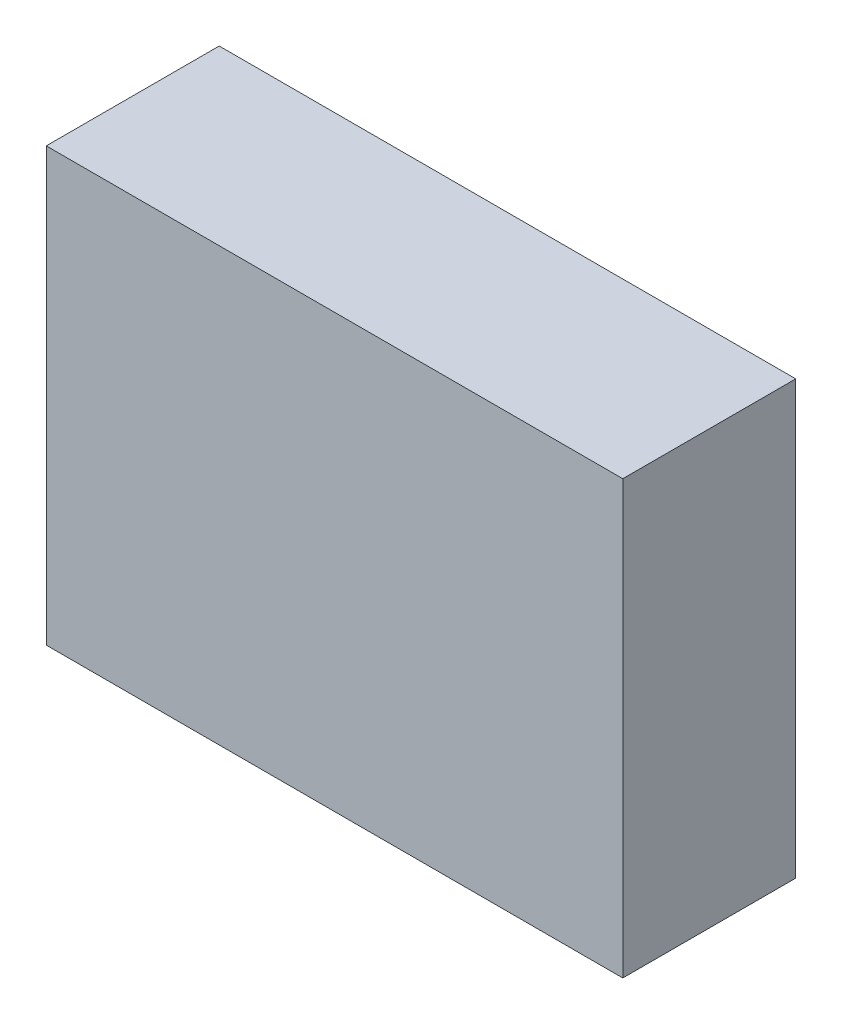
SolidWorks part; units mm, degrees
ref_plane "前视基准面" through (0, 0, 0) normal (0, 0, 1) x (1, 0, 0)
ref_plane "上视基准面" through (0, 0, 0) normal (0, 1, 0) x (1, 0, 0)
ref_plane "右视基准面" through (0, 0, 0) normal (1, 0, 0) x (0, 0, -1)
sketch "草图1" plane through (0, 0, 0) normal (0, 0, 1) x (1, 0, 0)
  line L1 (-20, -15) -> (20, -15)
  line L2 (-20, -15) -> (-20, 15)
  line L3 (-20, 15) -> (20, 15)
  line L4 (20, -15) -> (20, 15)
  line L5 (-20, -15) -> (20, 15) construction
  line L6 (-20, 15) -> (20, -15) construction
  point P0 (0, 0)
  dimension "D1" = 40
  dimension "D2" = 30
extrude "凸台-拉伸1" add sketch "草图1" along normal mid plane 12
